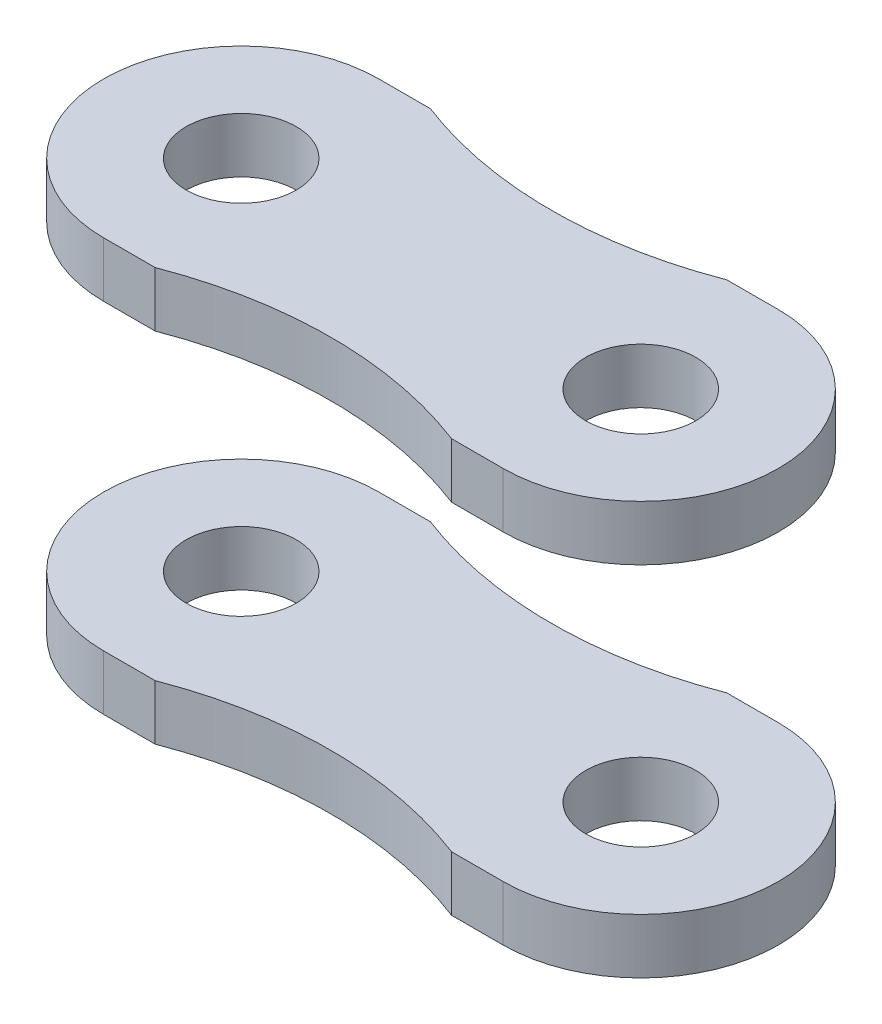
from build123d import *

# Parameters (mm, degrees)
SKETCH1_R               = 2
BOSS_EXTRUDE1_DEPTH     = 15
CUT_EXTRUDE1_DEPTH      = 5.5
CUT_EXTRUDE1_DEPTH_BACK = 5.5
SKETCH4_R               = 15
CUT_EXTRUDE2_DEPTH      = 15


with BuildPart() as part:
    # Sketch1 → Boss-Extrude1 (new body)
    with BuildSketch(Plane(origin=(0, 0, 0), x_dir=(1, 0, 0), z_dir=(0, 1, 0))):
        with BuildLine():
            Line((0, 5), (14.52, 5))
            ThreePointArc((14.52, 5), (19.52, 0), (14.52, -5))
            Line((14.52, -5), (0, -5))
            ThreePointArc((0, -5), (-5, 0), (0, 5))
        make_face()
        with Locations(Location((0, 0, 0), (0, 0, 270))):
            Circle(SKETCH1_R, mode=Mode.SUBTRACT)
        with Locations(Location((14.52, 0, 0), (0, 0, 270))):
            Circle(SKETCH1_R, mode=Mode.SUBTRACT)
    extrude(amount=BOSS_EXTRUDE1_DEPTH)

    # Sketch2 → Cut-Extrude1 (cut, two sides: drawn at the far end of the back side and taken through both)
    with BuildSketch(Plane(origin=(0, 7.5, 0), x_dir=(1, 0, 0), z_dir=(0, 1, 0)).offset(-CUT_EXTRUDE1_DEPTH_BACK)):
        with BuildLine():
            Line((0, 6.90174959), (14.52, 6.90174959))
            ThreePointArc((14.52, 6.90174959), (21.42174959, 0), (14.52, -6.90174959))
            Line((14.52, -6.90174959), (0, -6.90174959))
            ThreePointArc((0, -6.90174959), (-6.90174959, 0), (0, 6.90174959))
        make_face()
    extrude(amount=CUT_EXTRUDE1_DEPTH + CUT_EXTRUDE1_DEPTH_BACK, mode=Mode.SUBTRACT)


with BuildPart() as cut_extrude1_piece_1:
    # of the separate pieces the step leaves, piece 1, a body of its own (cut_extrude1_pieces)
    add(part.part.solids().sort_by_distance((14.52, 0, 5))[0])


with BuildPart() as cut_extrude1_piece_2:
    # of the separate pieces the step leaves, piece 2, a body of its own (cut_extrude1_pieces)
    add(part.part.solids().sort_by_distance((0, 13, 5))[0])


with BuildPart() as cut_extrude2_tool:
    # Sketch4 → Cut-Extrude2 (new body)
    with BuildSketch(Plane(origin=(0, 15, 0), x_dir=(1, 0, 0), z_dir=(0, 1, 0))):
        with Locations((7.26, 19)):
            Circle(SKETCH4_R)
        with Locations((7.26, -19)):
            Circle(SKETCH4_R)
    extrude(amount=-CUT_EXTRUDE2_DEPTH)


with BuildPart() as cut_extrude1_piece_1_1:
    add(cut_extrude1_piece_1.part)

    # Cut-Extrude2: cut by cut_extrude2_tool
    add(cut_extrude2_tool.part, mode=Mode.SUBTRACT)


with BuildPart() as cut_extrude1_piece_2_1:
    add(cut_extrude1_piece_2.part)

    # Cut-Extrude2: cut by cut_extrude2_tool
    add(cut_extrude2_tool.part, mode=Mode.SUBTRACT)


solid = Compound([cut_extrude1_piece_1_1.part, cut_extrude1_piece_2_1.part])
